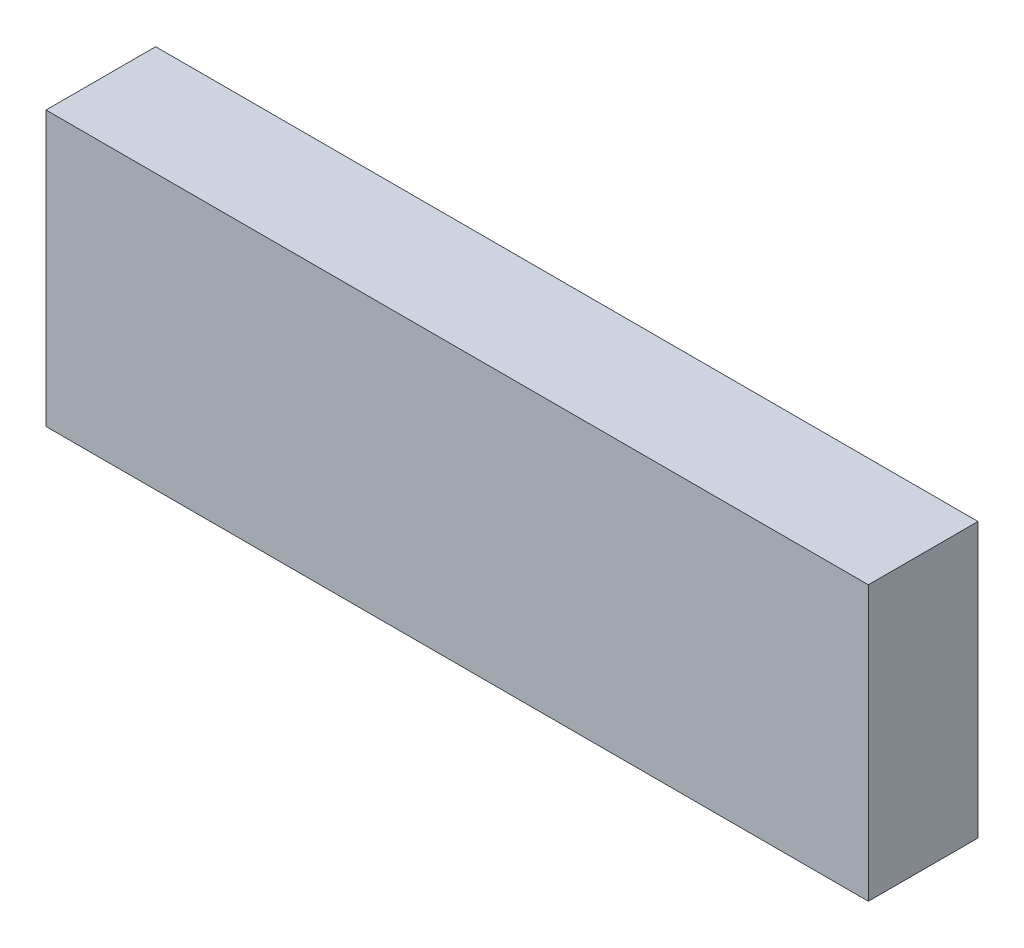
from build123d import *

# Parameters (mm, degrees)
SKETCH1_W           = 120
SKETCH1_H           = 40
BOSS_EXTRUDE1_DEPTH = 8


with BuildPart() as part:
    # Sketch1 → Boss-Extrude1 (new, symmetric)
    with BuildSketch(Plane.XY):
        Rectangle(SKETCH1_W, SKETCH1_H)
    extrude(amount=BOSS_EXTRUDE1_DEPTH, both=True)


solid = part.part
